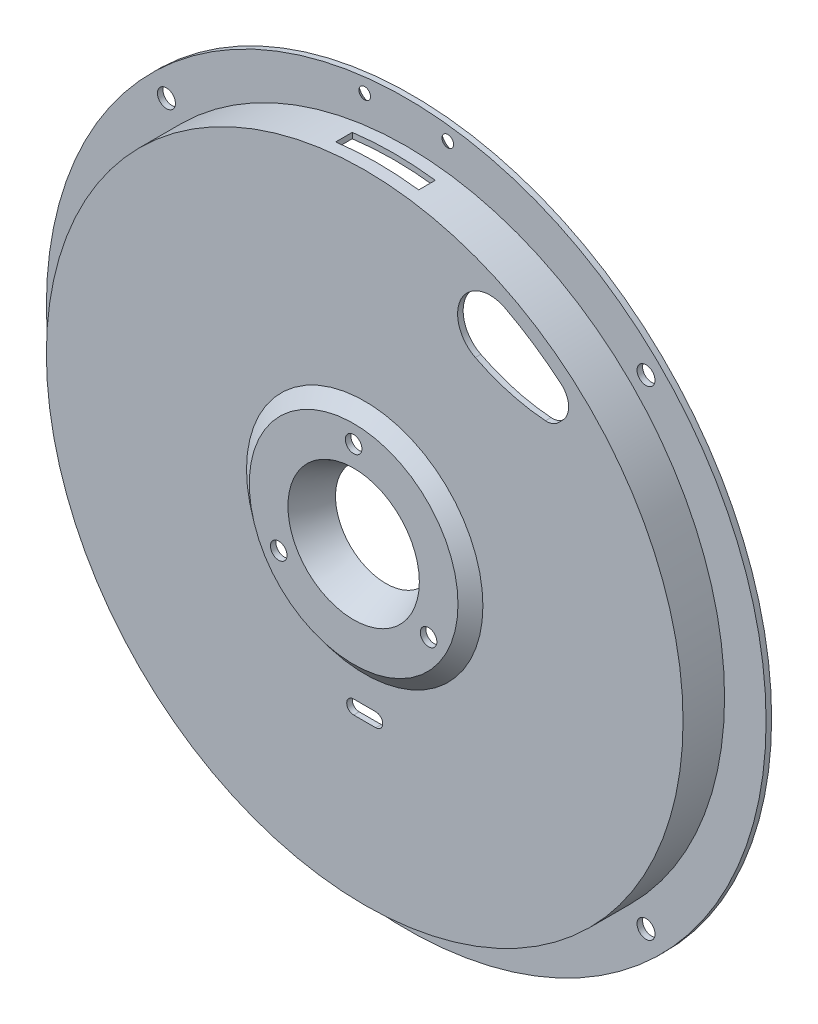
SolidWorks part; units mm, degrees
material "AISI 304"
ref_plane "Front Plane" through (0, 0, 0) normal (0, 0, 1) x (1, 0, 0)
ref_plane "Top Plane" through (0, 0, 0) normal (0, 1, 0) x (1, 0, 0)
ref_plane "Right Plane" through (0, 0, 0) normal (1, 0, 0) x (0, 0, -1)
sketch "Sketch1" plane through (0, 0, 0) normal (0, 1, 0) x (1, 0, 0)
  line L0 (-115, 15) -> (-130, 15)
  line L1 (-115, 0) -> (-42.7016, 0)
  line L2 (-67.4006, 2) -> (-113, 2)
  line L3 (-115, 0) -> (-115, 15)
  line L4 (0, 0) -> (-42.7016, 0) construction
  line L5 (-113, 17) -> (-130, 17)
  line L6 (-20, 8.5) -> (-18.1943, 7.6401)
  line L7 (-113, 2) -> (-113, 17)
  line L8 (-67.4006, 2) -> (-42, 2)
  line L9 (-42, 2) -> (-37, -2)
  line L10 (-37, -2) -> (-25, -2)
  line L11 (-130, 17) -> (-130, 15)
  line L12 (-25, -2) -> (-20, 8.5)
  line L13 (0, 0) -> (0, 42.3386) construction
  line L21 (-42.7016, 0) -> (-37.7016, -4)
  line L22 (-37.7016, -4) -> (-23.7372, -4)
  line L23 (-23.7372, -4) -> (-18.1943, 7.6401)
  point P25 (-55.5956, 0)
  dimension "D8" = 130
  dimension "D9" = 5
  dimension "D10" = 2
  dimension "D11" = 2
  dimension "D2" = 115
  dimension "D3" = 15
  dimension "D4" = 2
  dimension "D5" = 6.5
  dimension "D6" = 20
  dimension "D7" = 2
  dimension "D12" = 2
  dimension "D13" = 42
  dimension "D14" = 12
  dimension "D15" = 2
  dimension "D16" = 2
  dimension "D17" = 2
revolve "Revolve1" add sketch "Sketch1" angle 360 about L13
sketch "Sketch3" plane through (0, 0, -17) normal (0, 0, -1) x (-1, 0, 0)
  line L0 (-69.9774, 70.9471) -> (-71.467, 72.4368)
  line L2 (0, 0) -> (0, 81.6329) construction
  arc A0 (-69.9774, 70.9471) -> (-65.2951, 69.2059) centre (-65.7348, 75.1898) ccw
  arc A3 (-50.7076, 97.1463) -> (-71.0247, 83.4515) centre (0, 0) ccw
  arc A4 (-65.2951, 69.2059) -> (-39.9389, 76.3092) centre (-70.1564, 135.3667) ccw
  arc A5 (-50.7076, 97.1463) -> (-39.9389, 76.3092) centre (-45.2809, 86.7497) cw
  arc A6 (-71.467, 72.4368) -> (-71.0247, 83.4515) centre (-66.1637, 77.7401) cw
  point P3 (-77.0012, 77.971)
  point P9 (-66.3946, 67.3644)
  dimension "D2" = 15
  dimension "D3" = 7.5
  dimension "D4" = 6
extrude "Cut-Extrude1" cut sketch "Sketch3" against normal blind 45
sketch "Sketch4" plane through (0, 0, -2) normal (0, 0, -1) x (-1, 0, 0)
  line L0 (0, 0) -> (0, -55) construction
  line L1 (-4, -55) -> (4, -55) construction
  line L2 (-4, -52.5) -> (4, -52.5)
  line L3 (-4, -57.5) -> (4, -57.5)
  arc A0 (-4, -52.5) -> (-4, -57.5) centre (-4, -55) ccw
  arc A1 (4, -57.5) -> (4, -52.5) centre (4, -55) ccw
  point P5 (0, -55)
  dimension "D1" = 2.5
  dimension "D2" = 8
  dimension "D3" = 55
extrude "Cut-Extrude2" cut sketch "Sketch4" against normal blind 10
ref_plane "Plane1" through (0, 140, 0) normal (0, 1, 0) x (1, 0, 0)
sketch "Sketch5" plane through (0, 140, 0) normal (0, 1, 0) x (1, 0, 0)
  line L0 (0, 0) -> (0, 15) construction
  line L1 (-115, 15) -> (115, 15) construction
  line L3 (-15, 10.5) -> (15, 10.5)
  line L4 (-15, 10.5) -> (-15, 4.5)
  line L5 (-15, 4.5) -> (15, 4.5)
  line L6 (15, 10.5) -> (15, 4.5)
  line L7 (-15, 10.5) -> (15, 4.5) construction
  line L8 (-15, 4.5) -> (15, 10.5) construction
  point P5 (0, 7.5)
  dimension "D1" = 30
  dimension "D2" = 6
extrude "Cut-Extrude3" cut sketch "Sketch5" against normal blind 32
sketch "Sketch6" plane through (0, 0, -17) normal (0, 0, -1) x (-1, 0, 0)
  line L0 (0, 0) -> (0, 124) construction
  line L1 (-15, 124) -> (15, 124) construction
  dimension "D1" = 30
  dimension "D2" = 124
hole_wizard "Hole size by cross-recess countersunk self-tapping screw type1" positions "3DSketch1" profile "Sketch7" countersink size "ST3.5" standard "Gb" end condition through all
sketch3d "3DSketch1"
  point P0 (15, 124, -17)
  point P3 (-15, 124, -17)
sketch "Sketch7" plane through (15, 124, -17) normal (1, 0, 0) x (0, 1, 0)
  line L0 (0, 0) -> (0, 21)
  line L1 (0, 21) -> (1.85, 21)
  line L2 (1.85, 21) -> (1.85, 2.25)
  line L3 (1.85, 2.25) -> (4.1, 0)
  line L5 (4.1, 0) -> (0, 0)
  line L6 (-1.85, 2.25) -> (-4.1, 0) construction
  line L11 (0, -6.35) -> (0, 107.95) construction
  dimension "通孔孔直径" = 3.7
  dimension "通孔孔深度" = 21
  dimension "近端锥形沉头孔直径" = 8.2
  dimension "近端锥形沉头孔角度" = 90
sketch "Sketch8" plane through (0, 0, -17) normal (0, 0, -1) x (-1, 0, 0)
  line L0 (0, 0) -> (113.1646, 113.1646) construction
  line L1 (0, 0) -> (130, 0) construction
  circle A0 centre (0, 0) radius 130 construction
  circle A1 centre (0, 0) radius 122.5 construction
  circle A2 centre (86.6206, 86.6206) radius 3.25
  dimension "D2" = 245
  dimension "D3" = 6.5
  dimension "D1" = 45
extrude "Cut-Extrude4" cut sketch "Sketch8" against normal through all
pattern_circular "CirPattern1" count 4 over 360 about axis through (0, 0, 0) along (0, 0, 1) of "Cut-Extrude4"
sketch "Sketch9" plane through (0, 0, 2) normal (0, 0, -1) x (-1, 0, 0)
  circle A0 centre (0, 0) radius 31.25 construction
  circle A1 centre (0, 31.25) radius 3
  dimension "D1" = 62.5
  dimension "D2" = 6
extrude "Cut-Extrude5" cut sketch "Sketch9" against normal blind 28
pattern_circular "CirPattern2" count 3 over 360 about axis through (0, 0, 0) along (0, 0, 1) of "Cut-Extrude5"
